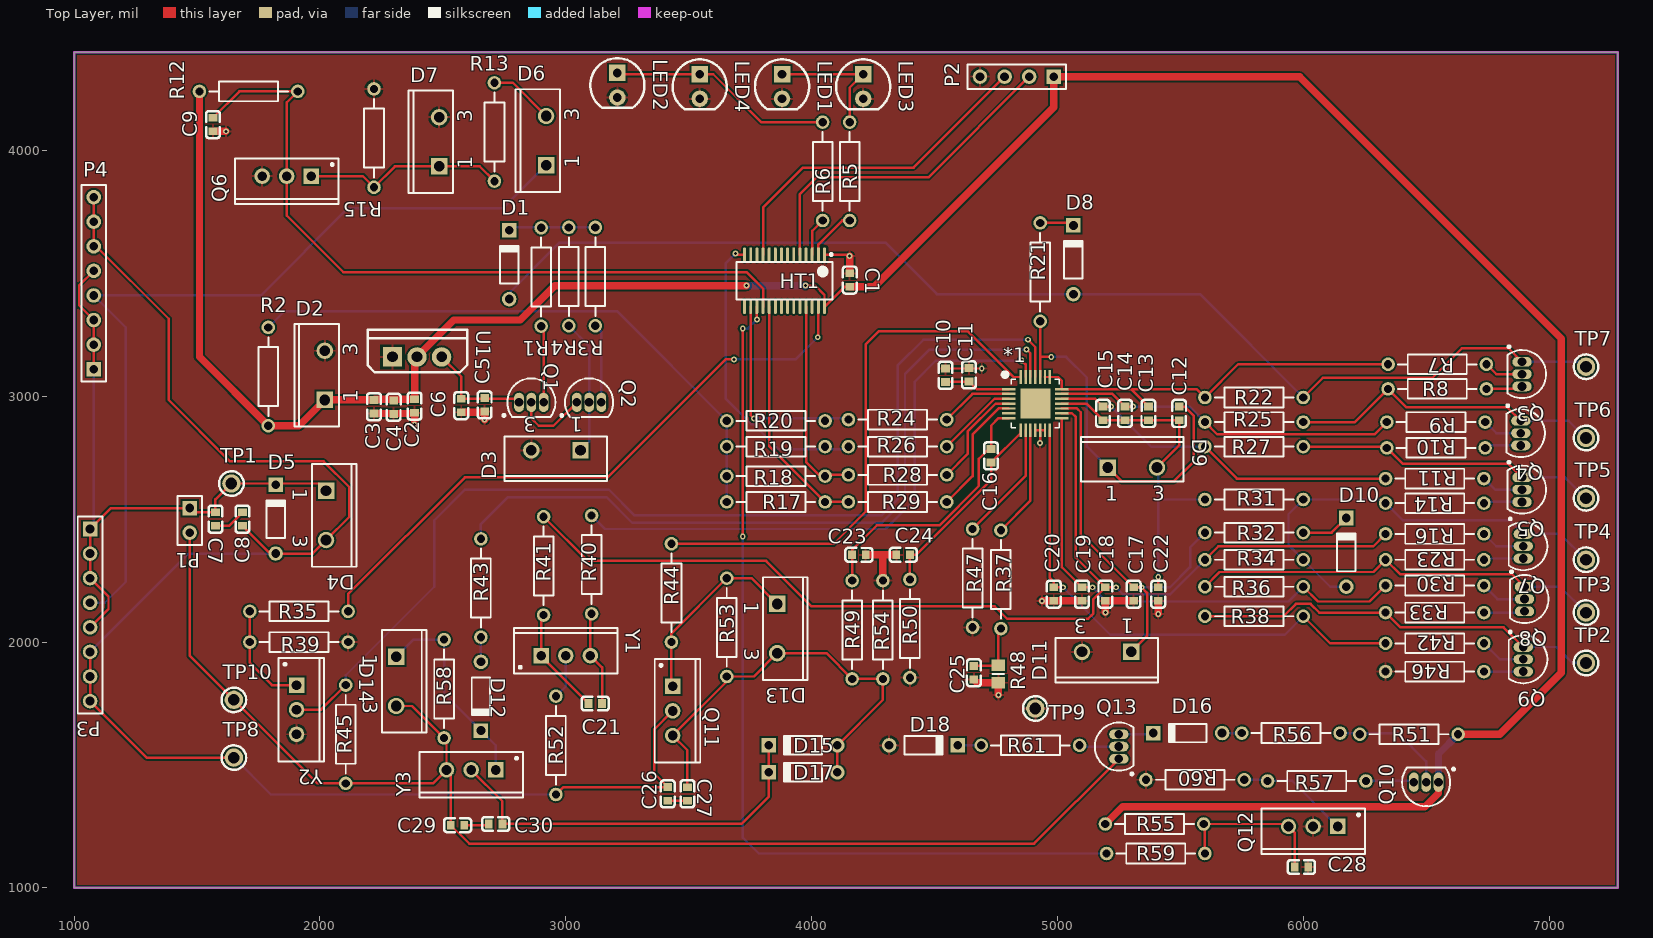
[diagram p0: Top Layer view]
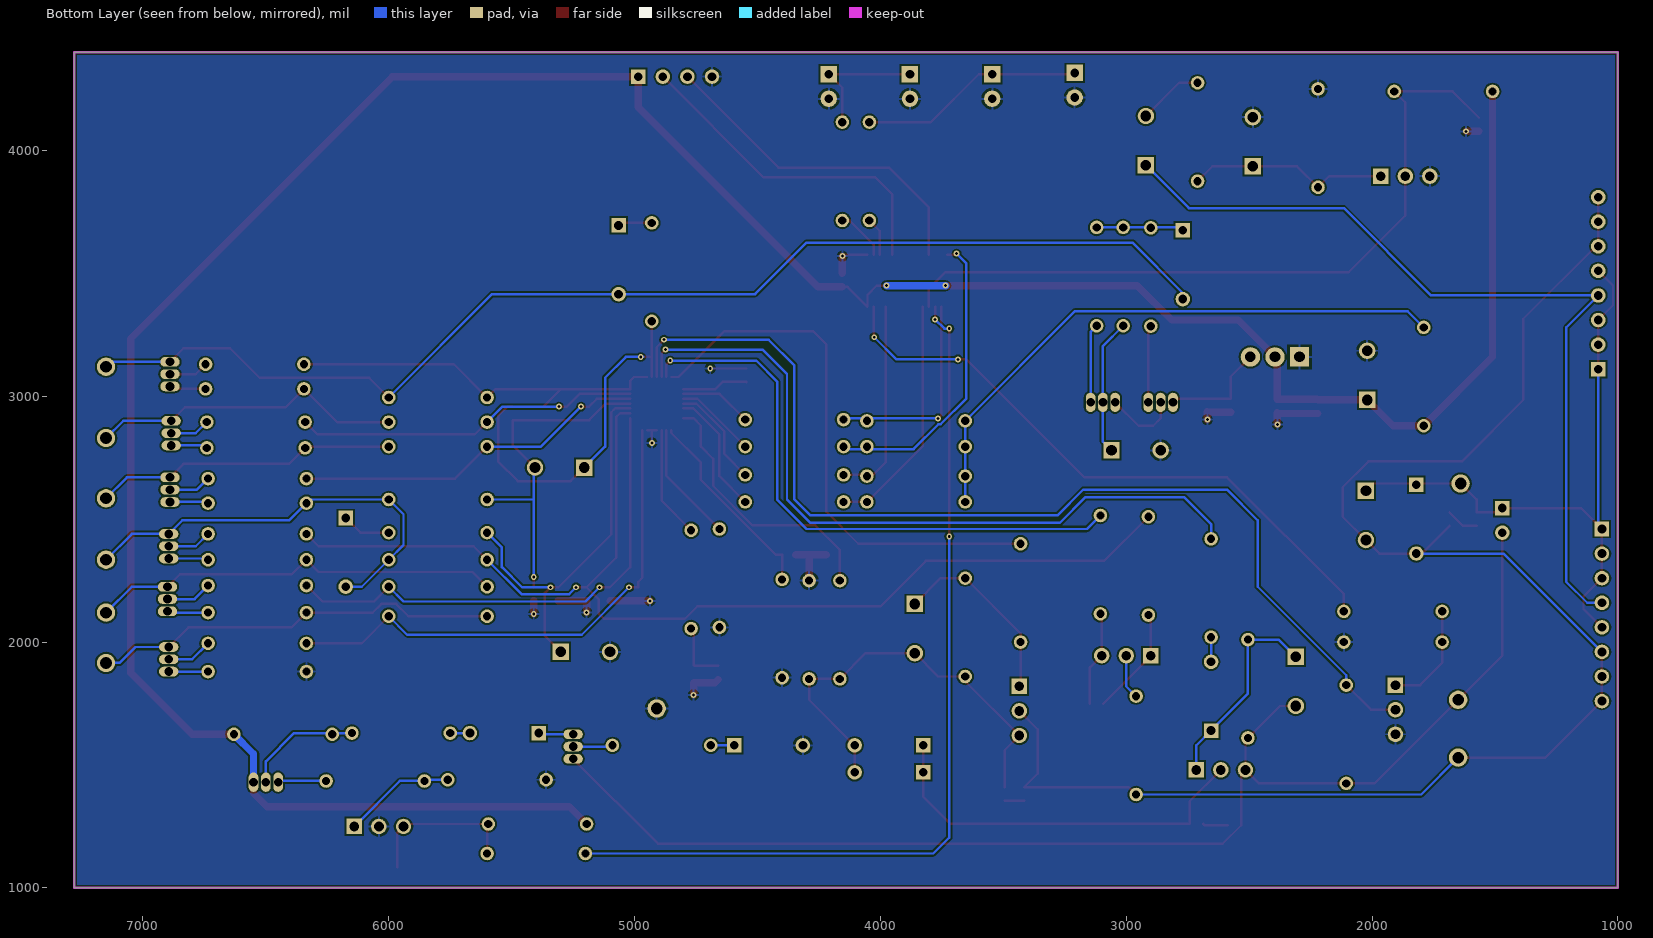
[diagram p1: Bottom Layer view, seen from below]
# Altium PCB MISC82104.PcbDoc
Units mil, origin at the board's own origin, x right, y up, seen from the top; angles counter-clockwise.
Board outline 6280 x 3400 mil, 2 copper layers (Top Layer, Bottom Layer); 146 components, 91 nets, 366 pads, 30 vias.

## Layer stack, top to bottom (the 12.6 mil dielectric is the usual default, probably not edited)
Top Solder: solder mask 0.4, Solder Resist, Dk 3.5
Top Layer: signal copper 1.4
Dielectric 1: dielectric 12.6, FR-4, Dk 4.8
Bottom Layer: signal copper 1.4
Bottom Solder: solder mask 0.4, Solder Resist, Dk 3.5

## Board outline
1000,1000 7280,1000 7280,4400 1000,4400

## Design rules (kind name [scope] priority, off if disabled: settings)
Clearance [All] p1: gap=7
MinimumSolderMaskSliver [All] p1: minsoldermaskwidth=0
PolygonConnect [All] p1: connectstyle=Relief reliefconductorwidth=10 reliefentries=4 polygonreliefangle="90 Angle" airgapwidth=10
RoutingVias [All] p1: holewidth=28 width=50 viastyle="Through Hole" minholewidth=28 minwidth=50 maxholewidth=28 maxwidth=50
SilkToSilkClearance [All] p1: silktosilkclearance=0
SilkToSolderMaskClearance [IsPad] p1: minsilkscreentomaskgap=0 clearancetoexposedcopper=TRUE
SolderMaskExpansion [All] p1: expansion=4
Width [All] p1: maxlimit=30 minlimit=10 preferedwidth=10
27 further rules are at their usual default settings.

## Components (designator, comment, footprint, x,y, rotation, side; value= is the part's Value field where it differs from the comment)
*1 "SH367306" QFN28L(5*5) 4910,2970 r0 top
C1 "104" C0603 4155.11,3472.75 r270 top
C2 "106" C0603 2385,2960 r90 top
C3 "NC" C0603 2219.89,2957.25 r90 top
C4 "104" C0603 2300,2955 r90 top
C5 "106" C0603 2670,2965 r90 top
C6 "104" C0603 2574.89,2962.14 r90 top
C7 "104" C0603 1575,2500 r90 top
C8 "104" C0603 1685,2500 r90 top
C9 "104" C0603 1565,4105 r90 top
C10 "104" C0603 4545,3085 r90 top
C11 "225" C0603 4639.89,3087.14 r90 top
C12 "225" C0603 5495,2930 r90 top
C13 "104" C0603 5370,2930 r90 top
C14 "104" C0603 5275,2930 r90 top
C15 "104" C0603 5185,2930 r90 top
C16 "104" C0603 4729.89,2757.25 r90 top
C17 "225" C0603 5310,2195 r90 top
C18 "104" C0603 5195,2195 r90 top
C19 "104" C0603 5099.89,2195 r90 top
C20 "104" C0603 4984.89,2195 r90 top
C21 "104" C0603 3120,1750 r0 top
C22 "225" C0603 5410,2195 r90 top
C23 "104" C0603 4192.75,2354.89 r180 top
C24 "104" C0603 4372.75,2354.89 r180 top
C25 "103" C0603 4660,1875 r90 top
C26 "104" C0603 3414.89,1382.25 r90 top
C27 "104" C0603 3495.11,1382.75 r270 top
C28 "103" C0603 5992.25,1085.11 r0 top
C29 "104" C0603 2560,1255 r180 top
C30 "104" C0603 2715,1260 r180 top
D1 "1N4148" DO-35 2770,3535 r90 top
D2 "MM3Z18" TO-220AC 2020,3085 r90 top
D3 "MM3Z18" TO-220AC 2960,2780 r180 top
D4 "MM3Z18" TO-220AC 2025,2515 r270 top
D5 "Diode 1N4148" DO-35 1820,2500 r90 top
D6 "MM3Z18" TO-220AC 2920,4040 r90 top
D7 "MM3Z18" TO-220AC 2485,4035 r90 top
D8 "Diode 1N4148" DO-35 5065,3555 r90 top
D9 "MM3Z18" TO-220AC 5305,2710 r0 top
D10 "Diode 1N4148" DO-35 6175,2365 r90 top
D11 "MM3Z18" TO-220AC 5200,1960 r180 top
D12 "1N4148" DO-35 2655,1780 r270 top
D13 "MM3Z18" TO-220AC 3860,2055 r270 top
D14 "MM3Z18" TO-220AC 2310,1840 r270 top
D15 "1N4148" DO-35 3965,1580 r180 top
D16 "1N4148" DO-35 5530,1630 r180 top
D17 "1N4148" DO-35 3965,1470 r180 top
D18 "1N4148" DO-35 4455,1580 r0 top
HT1 "HT66F3195" "SSOP28 - DUPLICATE" 3890,3470 r270 top
LED1 "I-LED" I-LED-5MM 3880,4310 r270 top
LED2 "I-LED" I-LED-5MM 3210,4315 r270 top
LED3 "I-LED" I-LED-5MM 4210,4310 r270 top
LED4 "I-LED" I-LED-5MM 3545,4310 r270 top
P1 "Header 2" HDR1X2 1470,2545 r270 top
P2 "Header 4" HDR1X4 4985,4300 r180 top
P3 "Header 8" HDR1X8 1065,2460 r270 top
P4 "Header 8" HDR1X8 1080,3110 r90 top
Q1 "2N3904" TO-92A 2860,2975 r270 top
Q2 "2N3904" TO-92A 3095,2975 r270 top
Q3 "2N3906" TO-92A 6890,3090 r180 top
Q4 "2N3906" TO-92A 6885,2850 r180 top
Q5 "2N3906" TO-92A 6890,2620 r180 top
Q6 "NMOS-2" TO-220AB 1865,3895 r180 top
Q7 "2N3906" TO-92A 6895,2390 r180 top
Q8 "2N3906" TO-92A 6900,2175 r180 top
Q9 "2N3906" TO-92A 6895,1930 r180 top
Q10 "2N3906" TO-92A 6500,1430 r90 top
Q11 "NMOS-2" TO-220AB 3435,1720 r270 top
Q12 "NMOS-2" TO-220AB 6040,1250 r180 top
Q13 "2N3904" TO-92A 5250,1575 r0 top
R1 "10" AXIAL-0.4 2900,3485 r270 top
R2 "NC" AXIAL-0.4 1790,3080 r90 top
R3 "104" AXIAL-0.4 3120.32,3486.56 r270 top
R4 "475" AXIAL-0.4 3012.44,3486.56 r270 top
R5 "621" AXIAL-0.4 4155,3915 r270 top
R6 "621" AXIAL-0.4 4045,3915 r270 top
R7 "511" AXIAL-0.4 6545,3130 r0 top
R8 "68" AXIAL-0.4 6545,3030 r180 top
R9 "511" AXIAL-0.4 6540,2895 r0 top
R10 "68" AXIAL-0.4 6540,2790 r180 top
R11 "511" AXIAL-0.4 6535,2665 r0 top
R12 "105" AXIAL-0.4 1710,4240 r180 top
R13 "205" AXIAL-0.4 2710,4075 r270 top
R14 "68" AXIAL-0.4 6535,2565 r180 top
R15 "205" AXIAL-0.4 2220,4050 r270 top
R16 "511" AXIAL-0.4 6535,2440 r0 top
R17 "103" AXIAL-0.4 3855,2570 r180 top
R18 "103" AXIAL-0.4 3855,2675 r180 top
R19 "103" AXIAL-0.4 3855,2795 r180 top
R20 "103" AXIAL-0.4 3855,2900 r180 top
R21 "51" AXIAL-0.4 4930,3505 r90 top
R22 "102" AXIAL-0.4 5800,2995 r0 top
R23 "68" AXIAL-0.4 6535,2335 r180 top
R24 "101" AXIAL-0.4 4350,2905 r0 top
R25 "102" AXIAL-0.4 5800,2895 r0 top
R26 "101" AXIAL-0.4 4350,2795 r0 top
R27 "102" AXIAL-0.4 5800,2795 r0 top
R28 "101" AXIAL-0.4 4350,2680 r0 top
R29 "101" AXIAL-0.4 4350,2570 r0 top
R30 "511" AXIAL-0.4 6535,2230 r0 top
R31 "101" AXIAL-0.4 5800,2580 r0 top
R32 "51" AXIAL-0.4 5800,2445 r0 top
R33 "68" AXIAL-0.4 6535,2120 r180 top
R34 "102" AXIAL-0.4 5800,2335 r0 top
R35 "101" AXIAL-0.4 1915,2125 r180 top
R36 "102" AXIAL-0.4 5800,2225 r180 top
R37 "101" AXIAL-0.4 4770,2255 r90 top
R38 "102" AXIAL-0.4 5800,2105 r180 top
R39 "105" AXIAL-0.4 1915,2000 r180 top
R40 "102" AXIAL-0.4 3105,2315 r90 top
R41 "102" AXIAL-0.4 2910,2310 r90 top
R42 "511" AXIAL-0.4 6535,1995 r0 top
R43 "102" AXIAL-0.4 2655,2220 r90 top
R44 "102" AXIAL-0.4 3430,2200 r90 top
R45 "105" AXIAL-0.4 2105,1625 r90 top
R46 "68" AXIAL-0.4 6535,1880 r180 top
R47 "101" AXIAL-0.4 4655,2260 r90 top
R48 "Res Varistor" 6-0805_N 4760,1870 r90 top
R49 "101" AXIAL-0.4 4165,2050 r90 top
R50 "101" AXIAL-0.4 4400,2055 r90 top
R51 "104" AXIAL-0.4 6430,1625 r0 top
R52 "104" AXIAL-0.4 2960,1580 r90 top
R53 "106" AXIAL-0.4 3655,2060 r90 top
R54 "101" AXIAL-0.4 4290,2050 r270 top
R55 "103" AXIAL-0.4 5395,1260 r0 top
R56 "104" AXIAL-0.4 5950,1630 r0 top
R57 "102" AXIAL-0.4 6055,1435 r0 top
R58 "104" AXIAL-0.4 2505,1810 r90 top
R59 "102" AXIAL-0.4 5400,1140 r180 top
R60 "105" AXIAL-0.4 5560,1440 r180 top
R61 "683" AXIAL-0.4 4890,1580 r180 top
TP1 "TP-RED" TEST-TH_BD2.54-P1.4_RED 1640,2645 r0 top
TP2 "TP-RED" TEST-TH_BD2.54-P1.4_RED 7150,1915 r0 top
TP3 "TP-RED" TEST-TH_BD2.54-P1.4_RED 7150,2120 r0 top
TP4 "TP-RED" TEST-TH_BD2.54-P1.4_RED 7150,2335 r0 top
TP5 "TP-RED" TEST-TH_BD2.54-P1.4_RED 7150,2585 r0 top
TP6 "TP-RED" TEST-TH_BD2.54-P1.4_RED 7150,2830 r0 top
TP7 "TP-RED" TEST-TH_BD2.54-P1.4_RED 7150,3120 r0 top
TP8 "TP-RED" TEST-TH_BD2.54-P1.4_RED 1650,1530 r0 top
TP9 "TP-RED" TEST-TH_BD2.54-P1.4_RED 4910,1730 r0 top
TP10 "TP-RED" TEST-TH_BD2.54-P1.4_RED 1650,1765 r90 top
U1 "LM317" TO220A 2395,3160 r0 top
Y1 "NMOS-2" TO-220AB 3000,1945 r0 top
Y2 "NMOS-2" TO-220AB 1905,1725 r270 top
Y3 "NMOS-2" TO-220AB 2615,1480 r180 top

## Footprints (in the part's own frame and the unit in brackets; to place one, negate y for a bottom-side part, rotate by r counter-clockwise, add the part's x,y. Pads: shape width x height; smd on the part's side, far side on the other; paste and mask are expansions set on the pad)
6-0805_N [mm] "Chip Resistor, Body 2.0x1.2mm, IPC Medium Density"
  rect 1.2x1.4 smd: 1(-0.9,0) 2(0.9,0)
  silkscreen extent 0,-0.6 0,0.6, body extent -1.07,-0.7 1.07,0.7, height 0.7
AXIAL-0.4 [mm] "Axial Device, Thru-Hole; 2 Leads; 0.4 in Pin Spacing"
  round 1.4 hole 0.85: 1(-5.08,0) 2(5.08,0)
  silkscreen extent -4.06,-1.02 4.06,1.02
C0603 [mm]
  rect 0.8x0.9 smd paste+0 mask+0.051: 1(-0.692,-0.003) 2(0.708,-0.003)
  silkscreen extent -1.4,-0.71 1.4,0.71
DO-35 [mm] "Diode, Axial; Body 3.8 x 1.9 mm (LxDia. max), Lead Dia. 0.53 mm (max)"
  round 1.5 hole 0.9: 1(-3.55,0)
  rect 1.5x1.5 hole 0.9: 2(3.55,0)
  silkscreen extent -1.95,-0.95 2.05,0.95
HDR1X2 [mm] "Connector; Header; 2 Position"
  rect 1.5x1.5 hole 0.9: 1(0,0)
  round 1.5 hole 0.9: 2(2.54,0)
  silkscreen extent -1.27,-1.27 3.81,1.27
HDR1X4 [mm] "Connector; Header; 4 Position"
  rect 1.5x1.5 hole 0.9: 1(0,0)
  round 1.5 hole 0.9: 2(2.54,0) 3(5.08,0) 4(7.62,0)
  silkscreen extent -1.27,-1.27 8.89,1.27
HDR1X8 [mm] "Connector; Header; 8 Position"
  rect 1.5x1.5 hole 0.9: 1(0,0)
  round 1.5 hole 0.9: 2(2.54,0) 3(5.08,0) 4(7.62,0) 5(10.16,0) 6(12.7,0) 7(15.24,0) 8(17.78,0)
  silkscreen extent -1.27,-1.27 19.05,1.27
I-LED-5MM [mm]
  rect 1.7x1.7 hole 0.9: 1(0,0)
  round 1.7 hole 0.9: 2(2.54,0)
  silkscreen extent -1.53,-2.8 3.6,2.8
QFN28L(5*5) [mm]
  rect 1.4x0.25 smd paste+0 mask+0.051: 1(-2.75,1.5) 2(-2.75,1) 3(-2.75,0.5) 4(-2.75,0) 5(-2.75,-0.5) 6(-2.75,-1) 7(-2.75,-1.5) 15(2.75,-1.5) 16(2.75,-1) 17(2.75,-0.5) 18(2.75,0) 19(2.75,0.5) 20(2.75,1) 21(2.75,1.5)
  rect 0.25x1.4 smd paste+0 mask+0.051: 8(-1.5,-2.75) 9(-1,-2.75) 10(-0.5,-2.75) 11(0,-2.75) 12(0.5,-2.75) 13(1,-2.75) 14(1.5,-2.75) 22(1.5,2.75) 23(1,2.75) 24(0.5,2.75) 25(0,2.75) 26(-0.5,2.75) 27(-1,2.75) 28(-1.5,2.75)
  rect 3.1x3.1 smd paste+0 mask+0.051: 29(0,0)
  silkscreen extent -3.25,-2.5 2.5,3.13
"SSOP28 - DUPLICATE" [mm]
  oval 1.5x0.3 smd paste+0 mask+0.051: 1(-2.7,4.128) 2(-2.7,3.493) 3(-2.7,2.858) 4(-2.7,2.223) 5(-2.7,1.588) 6(-2.7,0.953) 7(-2.7,0.318) 8(-2.7,-0.317) 9(-2.7,-0.952) 10(-2.7,-1.587) 11(-2.7,-2.222) 12(-2.7,-2.857) 13(-2.7,-3.492) 14(-2.7,-4.127) 15(2.7,-4.127) 16(2.7,-3.492) 17(2.7,-2.857) 18(2.7,-2.222) 19(2.7,-1.587) 20(2.7,-0.952) 21(2.7,-0.317) 22(2.7,0.318) 23(2.7,0.953) 24(2.7,1.588) 25(2.7,2.223) 26(2.7,2.858) 27(2.7,3.493) 28(2.7,4.128)
  silkscreen extent -2.83,-4.95 1.95,4.95
TEST-TH_BD2.54-P1.4_RED [mm]
  round 1.9 hole 1.2 paste+0 mask+0.051: 1(0,0)
  silkscreen extent -1.27,-1.27 1.27,1.27
TO220A [mm] "220，3脚晶体管"
  rect 2x2 hole 1.1: 1(-2.54,0)
  round 2 hole 1.1: 2(0,0) 3(2.54,0)
  silkscreen extent -5.08,-1.6 5.21,2.82, body extent -5.08,-1.45 5.22,2.98, height 18.5
TO-92A [mm] "TO, Flat Index; 3 In-Line, Axial Leads; Body Dia. 4.5mm; Leads 0.51 x 0.48 mm (max)"
  oval 2x1 hole 0.9: 1(0,-1.27) 2(0,0) 3(0,1.27)
  silkscreen extent -2.48,-2.95 1.5,2.48, body extent -2.48,-2.5 1.5,2.5, height 6.86
TO-220AB [mm] "TO, Thru-Hole, Vertical, Heatsink Mounted; 3 In-Line Leads; Pitch 2.54 mm"
  rect 1.6x1.6 hole 1: 1(-2.54,0)
  round 1.6 hole 1: 2(0,0) 3(2.54,0)
  silkscreen extent -5.35,-1.85 5.35,2.85, body extent -5.4,-1.9 5.4,2.9, height 19.3
TO-220AC [mm] "TO, Thru-Hole, Vertical, Heatsink Mounted; 3 In-Line Leads (1 Absent); Pitch 2.54 mm"
  rect 1.7x1.7 hole 1.1: 1(-2.54,0)
  round 1.7 hole 1.1: 3(2.54,0)
  silkscreen extent -5.3,-1.45 5.3,3.15

## Part data
C1 C2 C3 C4 C5 C6 C7 C8 C9 C10 C11 C12 C13 C14 C15 C16 C17 C18 C19 C20 C21 C22 C23 C24 C25 C26 C27 C28 C29 C30: library part Cap, "Capacitor"
D1 D12 D15 D16 D17 D18: library part "Diode 1N4148", "High Conductance Fast Diode"
D2 D3 D4 D6 D7 D9 D11 D13 D14: library part "Diode 10TQ045", "Schottky Rectifier"
D5 D8 D10: "High Conductance Fast Diode"
LED1 LED2 LED3 LED4: "Infrared diode"
P1: "Header, 2-Pin"
P2: "Header, 4-Pin"
P3 P4: "Header, 8-Pin"
Q1 Q2 Q13: "NPN General Purpose Amplifier"
Q3 Q4 Q5 Q7 Q8 Q9 Q10: "PNP General Purpose Amplifier"
Q6 Q11 Q12 Y1 Y2 Y3: "N-Channel Power MOSFET"
R1 R2 R3 R4 R5 R6 R7 R8 R9 R10 R11 R12 R13 R14 R15 R16 R17 R18 R19 R20 R21 R22 R23 R24 R25 R26 R27 R28 R29 R30 R31 R32 R33 R34 R35 R36 R37 R38 R39 R40 R41 R42 R43 R44 R45 R46 R47 R49 R50 R51 R52 R53 R54 R55 R56 R57 R58 R59 R60 R61: library part Res2, "Resistor"
R48: "Varistor (Voltage-Sensitive Resistor)"
U1: "Adjustable linear voltage regulator IC"

## Via types
v1: diameter 24, hole 12, Top Layer to Bottom Layer, 30 vias

## Nets (pads, with @x,y where several pads share a name; then routed paths per layer and width w, separated by ;. In a path a pad name is that pad's centre, name@x,y a point inside that pad or via, vN(x,y) a via of type N, cw(c..) or ccw(c..) an arc to the next point about the centre after c; other vN are vias at no path point)
AF_WAKE: HT1.27 R35.1 | length 2537.6
  Top Layer w10: R35.1 2115,2195 2590,2670 3170,2670 3650,3150 v1(3685,3150) ; v1(4025,3240) 4027.5,3242.5 HT1.27
  Bottom Layer w10: v1(3685,3150) 3935,3150 v1(4025,3240)
ALARM: HT1.19 R17.1 R29.1 | length 982.9
  Top Layer w10: HT1.19 3827.5,2797.5 R17.1 R29.1
B1: Q9.1 R33.2 R38.2 TP2.1 | length 1670.1
  Top Layer w10: R38.2 5920,2105 5970,2155 6030,2155 6065,2120 R33.2 6395,2060 6815,2060 Q9.1
  Bottom Layer w10: Q9.1 7030,1980 7095,1915 TP2.1
B2: Q8.1 R23.2 R36.2 TP3.1 | length 1684.6
  Top Layer w10: R36.2 5660,2285 6285,2285 R23.2 6395,2275 6850,2275 Q8.1
  Bottom Layer w10: Q8.1 7045,2225 TP3.1
B3: D10.1 Q7.1 R14.2 R31.2 R34.2 TP4.1 | length 1766.7
  Bottom Layer w10: D10.1 6109.76,2225.24 R34.2 5940,2395 5940,2520 R31.2 6320,2580 R14.2 6405,2495 6840,2495 Q7.1 7045,2440 TP4.1
B4: Q5.1 R10.2 R27.2 TP5.1 | length 1237
  Top Layer w10: R27.2 6335,2795 R10.2 6405,2725 6835,2725 Q5.1
  Bottom Layer w10: Q5.1 7065,2670 TP5.1
B5: Q4.1 R8.2 R25.2 TP6.1 | length 1288.8
  Top Layer w10: R25.2 6210,2895 R8.2 6420,2955 6830,2955 Q4.1
  Bottom Layer w10: Q4.1 7080,2900 TP6.1
B6: D1.1 D8.1 Q3.1 R22.2 TP7.1 | length 4892.8
  Top Layer w10: R22.2 6080,3075 6525,3075 6645,3195 6835,3195 Q3.1 ; TP7.1@7130,3140 TP7.1
  Bottom Layer w10: D1.1 2770,3420 2975,3625 4300,3625 4509.76,3415.24 D8.1 5579.76,3415.24 R22.2 ; Q3.1 7130,3140 TP7.1
C+: C7.2 D4.1 D5.2 P1.1 P3.1 P3.2 P3.3 P3.5 P4.1 P4.2 P4.3 P4.5 TP1.1 | length 2661.9
  Top Layer w10: P3.5 1140,2135 1140,2185 P3.3 P3.2 P3.1 1150,2545 P1.1 1487.14,2527.86 C7.2 1575.11,2580.11 TP1.1 1995,2645 D4.1 ; P4.1 P4.2 P4.3 1020,3370 1020,3450 P4.5
  Bottom Layer w10: P3.1 1080,2475 P4.1
C-: C29.2 D14.3 P1.2 Q13.1 R45.1 R58.1 TP10.1 Y3.3 | length 5290
  Top Layer w10: P1.2 1470,1945 TP10.1 1990,1425 R45.1 2460,1425 Y3.3 ; D14.3 2375,1740 R58.1 2515,1600 Y3.3 ; Q13.1 4905,1180 2607.24,1180 C29.2 2532.14,1462.86 Y3.3
CB1: *1.14 C20.2 R38.1 R42.1 | length 2152
  Top Layer w10: *1.14 4969.06,2260.95 4985,2245 C20.2 v1(5022.14,2222.86) ; R38.1 6110,1995 R42.1
  Bottom Layer w10: v1(5022.14,2222.86) 5215,2030 5925,2030 R38.1
CB2: *1.15 C19.2 R30.1 R36.1 | length 2057.5
  Top Layer w10: *1.15 5018.27,2304.6 C19.2 v1(5142.14,2222.86) ; R36.1 6060,2165 6270,2165 R30.1
  Bottom Layer w10: v1(5142.14,2222.86) 5200,2165 5940,2165 R36.1
CB3: *1.16 C18.2 R16.1 R34.1 R41.2 | length 4601.8
  Top Layer w10: R41.2 3090,2330 3815,2330 4000,2145 4745,2145 4795,2095 5125,2095 5145,2115 5145,2172.76 C18.2 ; *1.16 5059.37,2930.63 5075,2915 5075,2342.97 C18.2 ; v1(5237.86,2222.86) C18.2 ; R34.1 5655,2390 6285,2390 R16.1
  Bottom Layer w10: v1(5237.86,2222.86) 5265.73,2195 5460,2195 R34.1
CB4: *1.19 C15.2 R11.1 R27.1 | length 1451.2
  Top Layer w10: *1.19 5153.29,2989.68 C15.2 v1(5217.86,2957.86) ; R27.1 5730,2665 R11.1
  Bottom Layer w10: v1(5217.86,2957.86) 5380.73,2795 R27.1
CB5: *1.20 C14.2 R9.1 R25.1 | length 1410.5
  Top Layer w10: *1.20 5223.6,3009.37 C14.2 v1(5307.86,2957.86) ; R25.1 5650,2845 6290,2845 R9.1
  Bottom Layer w10: v1(5307.86,2957.86) 5537.14,2957.86 R25.1
CB6: *1.21 *1.22 *1.23 C13.2 R7.1 R22.1 | length 1605.9
  Top Layer w10: *1.23 *1.22 5001.73,3078.27 5018.27,3061.74 *1.21 5298.92,3029.05 ; C13.2 5298.92,3029.05 ; R7.1 5735,3130 R22.1 5565.95,3029.05 5298.92,3029.05
CHG: *1.26 R43.2 | length 3077.9
  Top Layer w10: v1(4875,3190) 4890.31,3174.68 *1.26
  Bottom Layer w10: R43.2 2655,2480 2765,2590 3165.44,2590 3270.44,2485 4285,2485 4380,2580 4380,3090 4480,3190 v1(4875,3190)
CHGD: *1.25 R45.2 Y2.2 | length 4350.4
  Top Layer w10: Y2.2 2005,1725 R45.2 ; v1(4880,3230) 4910.01,3199.99 *1.25
  Bottom Layer w10: R45.2 2105,1865 2465,2225 2465,2495 2590,2620 3175,2620 3280,2515 4285,2515 4350,2580 4350,3125 4455,3230 v1(4880,3230)
CS: HT1.17 R59.2 | length 3701.2
  Top Layer w10: v1(3720,2430) v1(3720,3275) ; v1(3777.5,3312.5) HT1.17
  Bottom Layer w10: v1(3720,2430) 3720,1205 3785,1140 R59.2 ; v1(3720,3275) 3740,3275 v1(3777.5,3312.5)
CTLD: HT1.25 R18.1 R28.1 | length 825.4
  Top Layer w10: HT1.25 3977.5,2732.5 4030,2680 R28.1
DSG: *1.28 R44.2 | length 2254.9
  Top Layer w10: R44.2 4090,2400 4220,2530 4220,3210 4275,3265 4635,3265 4821.73,3078.27 *1.28
DSGD: *1.27 R40.2 | length 2410.9
  Top Layer w10: v1(4855,3145) 4870.64,3129.36 *1.27
  Bottom Layer w10: R40.2 3160,2460 4300,2460 4420,2580 4420,3060 4505,3145 v1(4855,3145)
GND: *1.11 *1.12 *1.13 C1.1 C2.1 C3.1 C4.1 C5.1 C6.1 C9.1 C10.2 C11.2 C17.1 C18.1 C19.1 C20.1 C22.1 C23.1 C24.2 C25.1 C28.2 D2.3 D3.3 D7.3 D11.3 D18.1 HT1.1 LED1.2 LED2.2 LED3.2 LED4.2 P2.4 Q6.3 Q12.2 R15.1 R39.1 R46.2 R47.1 R48.1 R50.1 R54.1 R60.2 TP9.1 U1.1 Y2.3 | length 1571.9
  Top Layer w10: HT1.1 4148.7,3576.3 v1(4155,3570) ; C10.2 v1(4692.14,3112.86) ; *1.11 *1.12 ; v1(4929.69,2810.32) *1.12 ; *1.13 *1.12
  Top Layer w30: C9.1 v1(1617.75,4077.75) ; C3.1 2382.35,2930 C2.1 v1(2385.11,2884.89) ; C6.1 2667.24,2934.89 C5.1 v1(2670.11,2904.89) ; C1.1 v1(4155,3570) ; C23.1 4290,2355 ; R54.1 4290,2355 ; C24.2 4290,2355 ; C25.1 4673.29,1834.57 R48.1 v1(4760,1785) ; v1(4937.25,2167.75) C20.1 C19.1 ; v1(5195.11,2120.11) C18.1 C17.1 ; v1(5410.11,2114.89) C22.1
ICPCK: HT1.11 P2.3 | length 1394.3
  Top Layer w10: HT1.11 3802.5,3767.5 3965,3930 4415,3930 P2.3
ICPDA: HT1.5 P2.2 | length 1376.5
  Top Layer w10: HT1.5 3952.5,3822.5 4020,3890 4475,3890 P2.2
K: D6.1 P3.4 P4.4 | length 3458.6
  Bottom Layer w10: P3.4 1125,2160 1210,2245 1210,3280 P4.4 1760,3410 2115,3765 2745,3765 D6.1
LOAD: C9.2 HT1.18 Q6.2 R12.1 | length 3047.4
  Top Layer w10: C9.2 1672.24,4240 R12.1 1865,4195 Q6.2 1865,3735 2095,3505 3735,3505 3802.5,3437.5 HT1.18
Net*1_1: *1.1 C10.1 C11.1 | length 270.3
  Top Layer w10: C10.1 4547.24,3059.89 C11.1 4670.84,3029.05 *1.1
Net*1_2: *1.2 R24.2 | length 295
  Top Layer w10: R24.2 4654.37,3009.37 *1.2
Net*1_3: *1.3 R26.2 | length 332.4
  Top Layer w10: R26.2 4744.68,2989.68 *1.3
Net*1_4: *1.4 R28.2 | length 425.1
  Top Layer w10: R28.2 4635,2765 4635,2855.96 4749.04,2970 *1.4
Net*1_5: *1.5 R29.2 | length 508.8
  Top Layer w10: R29.2 4655,2675 4655,2845 4760.31,2950.31 *1.5
Net*1_7: *1.7 C16.2 C23.2 R49.2 | length 1098
  Top Layer w10: R49.2 4164.89,2250.11 C23.2 4164.89,2374.89 4265,2475 4520,2475 4680,2635 4680,2745 4730,2795 4730,2880 4760.94,2910.94 *1.7
Net*1_8: *1.8 C16.1 C24.1 R50.2 | length 808.2
  Top Layer w10: R50.2 C24.1 4425,2355 4730,2660 C16.1 4850.94,2850.95 *1.8
Net*1_9: *1.9 R47.2 | length 491
  Top Layer w10: R47.2 4870.64,2675.64 *1.9
Net*1_10: *1.10 R37.2 | length 456.6
  Top Layer w10: R37.2 4890.31,2575.32 *1.10
Net*1_18: *1.18 C12.1 C13.1 C14.1 C15.1 C22.2 D9.3 R31.1 | length 1413.9
  Top Layer w10: *1.18 5117.86,2970 C15.1 C14.1 C13.1 C12.1 5495.11,2800.11 D9.3 ; C22.2 v1(5410.11,2264.89)
  Bottom Layer w10: D9.3 5410.11,2704.89 5410.11,2580 ; v1(5410.11,2264.89) 5410.11,2580 ; R31.1 5410.11,2580
Net*1_24: *1.24 C12.2 D9.1 R21.1 | length 1529.1
  Top Layer w10: *1.24 4929.69,3160 ; R21.1 4929.69,3304.68 4929.69,3160 ; v1(4975,3160) 4929.69,3160 ; D9.1 5260,2655 5475,2655 5555,2735 5555,2920 5517.14,2957.86 C12.2
  Bottom Layer w10: v1@4965,3160 v1(4975,3160) 5035,3160 5120,3075 5120,2795 D9.1
NetC7_1: C7.1 C8.2 | length 132.8
  Top Layer w10: C7.1 1630,2472.75 C8.2
NetC21_1: C21.1 R41.1 Y1.1 | length 444.1
  Top Layer w10: R41.1 2900,2100 Y1.1 2900,1942.65 C21.1
NetC21_2: C21.2 R40.1 Y1.3 | length 387
  Top Layer w10: R40.1 3100,2110 Y1.3 3147.86,1897.14 C21.2
NetC25_2: C25.2 R37.1 R48.2 | length 254.7
  Top Layer w10: C25.2 4757.43,1902.86 R48.2 4760,2045 R37.1
NetC26_1: C26.1 C27.2 | length 80
  Top Layer w10: C26.1 3494.89,1355 C27.2
NetC27_1: C27.1 D13.3 D15.1 D17.1 Q11.3 R49.1 R53.1 R54.2 | length 1740.5
  Top Layer w10: C27.1 3495,1560 Q11.3 3655,1840 R53.1 3765,1860 D13.3 4060,1955 R49.1 R54.2 4290,1765.24 D15.1 D17.1
NetC28_1: C28.1 Q12.3 R55.2 R59.1 | length 646.6
  Top Layer w10: R59.1 5600,1255 R55.2 5930,1260 Q12.3 5965,1225 C28.1
NetC29_1: C29.1 C30.2 | length 102
  Top Layer w10: C29.1 2682.14,1255.11 C30.2
NetC30_1: C30.1 D15.2 D17.2 Y3.2 | length 1611
  Top Layer w10: Y3.2 2742.25,1352.75 C30.1 3715.11,1260.11 3825.24,1370.24 D17.2 D15.2
NetD1_2: D1.2 R1.1 R3.1 R4.1 | length 355.2
  Bottom Layer w10: D1.2 2781.8,3686.56 R4.1 R3.1
NetD3_1: D3.1 Q2.2 R4.2 | length 555.3
  Bottom Layer w10: R4.2 3095,3204 Q2.2 3095,2815 D3.1
NetD6_3: D6.3 R13.1 | length 265.9
  Top Layer w10: R13.1 2785,4275 D6.3
NetD7_1: D7.1 Q6.1 R13.2 R15.2 | length 823.7
  Top Layer w10: Q6.1 2175,3895 R15.2 2305,3935 D7.1 2650,3935 R13.2
NetD8_2: D8.2 R21.2 | length 139.2
  Top Layer w10: R21.2 5054.76,3705 D8.2
NetD10_2: D10.2 R32.2 | length 199.8
  Top Layer w10: R32.2 6115.24,2445 D10.2
NetD12_1: D12.1 R43.1 | length 100.2
  Bottom Layer w10: D12.1 R43.1
NetD12_2: D12.2 D14.1 R58.2 Y3.1 | length 841
  Bottom Layer w10: D14.1 2380,2010 R58.2 2505,1790.24 D12.2 2715,1580.24 Y3.1
NetD13_1: D13.1 Q11.1 R44.1 R53.2 | length 783.8
  Top Layer w10: Q11.1 3430,1825 R44.1 3430,2035 R53.2 3755,2260 D13.1
NetD16_1: D16.1 R56.1 | length 80.2
  Bottom Layer w10: D16.1 R56.1
NetD16_2: D16.2 Q13.3 | length 142.3
  Bottom Layer w10: Q13.3 5385.24,1625 D16.2
NetD18_2: D18.2 R61.2 | length 95.2
  Bottom Layer w10: D18.2 R61.2
NetHT1_2: HT1.2 R5.2 | length 209.1
  Top Layer w10: HT1.2 4027.5,3617.5 4125,3715 R5.2
NetHT1_3: HT1.3 R6.2 | length 156.3
  Top Layer w10: HT1.3 4002.5,3672.5 R6.2
NetLED1_1: LED1.1 LED3.1 R5.1 | length 547.8
  Top Layer w10: LED1.1 LED3.1 4155,4255 R5.1
NetLED2_1: LED2.1 LED4.1 R6.1 | length 917.8
  Top Layer w10: LED2.1 3215,4310 LED4.1 3600,4310 3795,4115 R6.1
NetQ1_2: Q1.2 Q2.1 | length 301.8
  Top Layer w10: Q1.2 2860,2910 2890,2880 2950,2880 Q2.1
NetQ1_3: Q1.3 R1.2 | length 314.1
  Top Layer w10: R1.2 2910,3275 Q1.3
NetQ2_3: Q2.3 R3.2 | length 321.8
  Bottom Layer w10: R3.2 3145,3261.87 Q2.3
NetQ3_2: Q3.2 R7.2 | length 161.6
  Top Layer w10: R7.2 6785,3090 Q3.2
NetQ3_3: Q3.3 R8.1 | length 149.1
  Top Layer w10: R8.1 6880,3030 Q3.3
NetQ4_2: Q4.2 R9.2 | length 163.6
  Bottom Layer w10: R9.2 6785,2850 Q4.2
NetQ4_3: Q4.3 R10.1 | length 149.1
  Bottom Layer w10: R10.1 6750,2800 Q4.3
NetQ5_2: Q5.2 R11.2 | length 173.6
  Bottom Layer w10: R11.2 6780,2620 Q5.2
NetQ5_3: Q5.3 R14.1 | length 157.1
  Bottom Layer w10: R14.1 6740,2570 Q5.3
NetQ7_2: Q7.2 R16.2 | length 180.7
  Bottom Layer w10: R16.2 6785,2390 Q7.2
NetQ7_3: Q7.3 R23.1 | length 162.1
  Bottom Layer w10: R23.1 6740,2340 Q7.3
NetQ8_2: Q8.2 R30.2 | length 187.8
  Bottom Layer w10: R30.2 6790,2175 Q8.2
NetQ8_3: Q8.3 R33.1 | length 167.1
  Bottom Layer w10: R33.1 6895,2120 Q8.3
NetQ9_2: Q9.2 R42.2 | length 186.9
  Bottom Layer w10: R42.2 6800,1930 Q9.2
NetQ9_3: Q9.3 R46.1 | length 160
  Bottom Layer w10: R46.1 Q9.3
NetQ10_2: Q10.2 R51.1 R56.2 | length 482.6
  Bottom Layer w10: R56.2 6385,1630 6500,1515 Q10.2
NetQ10_3: Q10.3 R57.2 | length 197.1
  Bottom Layer w10: R57.2 6445,1435 Q10.3
NetQ12_1: Q12.1 R57.1 R60.1 | length 458.7
  Bottom Layer w10: R60.1 5850,1440 R57.1 5955,1435 Q12.1
NetQ13_2: Q13.2 R61.1 | length 162.1
  Bottom Layer w10: R61.1 5095,1575 Q13.2
NetR35_2: R35.2 R39.2 Y2.1 | length 437.3
  Top Layer w10: R35.2 R39.2 1715,1915 1805,1825 Y2.1
NetR52_2: R52.2 Y1.2 | length 181.6
  Bottom Layer w10: R52.2 3000,1820 Y1.2
P-: C8.1 C26.2 D4.3 D5.1 P3.6 P3.7 P3.8 P4.6 P4.7 P4.8 Q11.2 R52.1 TP8.1 | length 6501.3
  Top Layer w10: P3.6 P3.7 P3.8 1295,1530 TP8.1 ; P4.8 P4.7 1080,3620 1385,3315 1385,2985 1635,2735 2015,2735 2120,2630 2120,2510 D4.3 1970.24,2360.24 D5.1 1797.62,2360.24 C8.1 ; R52.1 2990.11,1410.11 C26.2 3360,1465.11 3360,1645 Q11.2
  Bottom Layer w10: P3.6 1465.24,2360.24 D5.1 ; TP8.1 1800,1380 R52.1
SCL: HT1.14 R19.1 R26.1 | length 1234
  Top Layer w10: v1(3690,3580) 3693.7,3576.3 HT1.14
  Bottom Layer w10: v1(3690,3580) 3650,3540 3650,2991.06 3755.06,2886 3764,2886 3865,2785 4140,2785 R26.1
SDA: HT1.16 R20.1 R24.1 | length 845.9
  Top Layer w10: HT1.16 3752.5,2922.5 v1(3765,2910)
  Bottom Layer w10: v1(3765,2910) 4145,2910 R24.1
V11: C5.2 C6.2 Q1.1 U1.3 | length 444.4
  Top Layer w10: U1.3 2575,3080 C6.2 2795,2990 Q1.1
V33: R2.2 R17.2 R18.2 R19.2 R20.2 | length 2406.2
  Bottom Layer w10: R2.2 1855,3345 3210,3345 R20.2 R19.2 R18.2 R17.2
VCC: C1.2 C2.2 C3.2 C4.2 D2.1 HT1.28 P2.1 Q10.1 R2.1 R12.2 R51.2 R55.1 U1.2 | length 11597.1
  Top Layer w10: v1(3975,3450) 4015,3450 4052.5,3412.5 HT1.28 4133.69,3444.89 C1.2
  Top Layer w30: R12.2 1510,3160 R2.1 1915,2880 D2.1 2219.89,2985 C3.2 2222.75,2987.86 C2.2 2385.11,3150.11 U1.2 2545,3310 2815,3310 2955,3450 v1(3735,3450) ; C1.2 4254.89,3444.89 4985,4175 P2.1 5985,4300 7050,3235 7050,1875 6800,1625 R51.2 ; R55.1 5265,1330 6495,1330 6550,1385 Q10.1
  Bottom Layer w30: v1(3735,3450) v1(3975,3450) ; Q10.1 6550,1545 R51.2
VDD: *1.17 C17.2 D11.1 R32.1 | length 1612.3
  Top Layer w10: *1.17 5079.69,2950.31 5095,2935 5095,2437.97 C17.2 v1(5342.14,2222.86) 5365,2200 5365,2025 D11.1
  Bottom Layer w10: v1(5342.14,2222.86) 5457.86,2222.86 5540,2305 5540,2385 R32.1
pads on no net: *1.6 *1.29 HT1.4 HT1.6 HT1.7 HT1.8 HT1.9 HT1.10 HT1.12 HT1.13 HT1.15 HT1.20 HT1.21 HT1.22 HT1.23 HT1.24 HT1.26

## Polygon pours and split planes (outlines as drawn)
GND on Top Layer "G" (solid, remove dead copper, pour order 0): 605,4945 935,4615 7720,4615 7720,760 7920,560 7825,655 815,655
GND on Bottom Layer "G" (solid, remove dead copper, pour order 2): 40,4845 8520,4845 8665,4700 7665,3700 7665,405 970,405 700,675

## Keep-outs
Keep-Out Layer:
  lines w10: 1000,1000 1000,4400 4750,4400 7280,4400 7280,3275 7280,1000 1000,1000